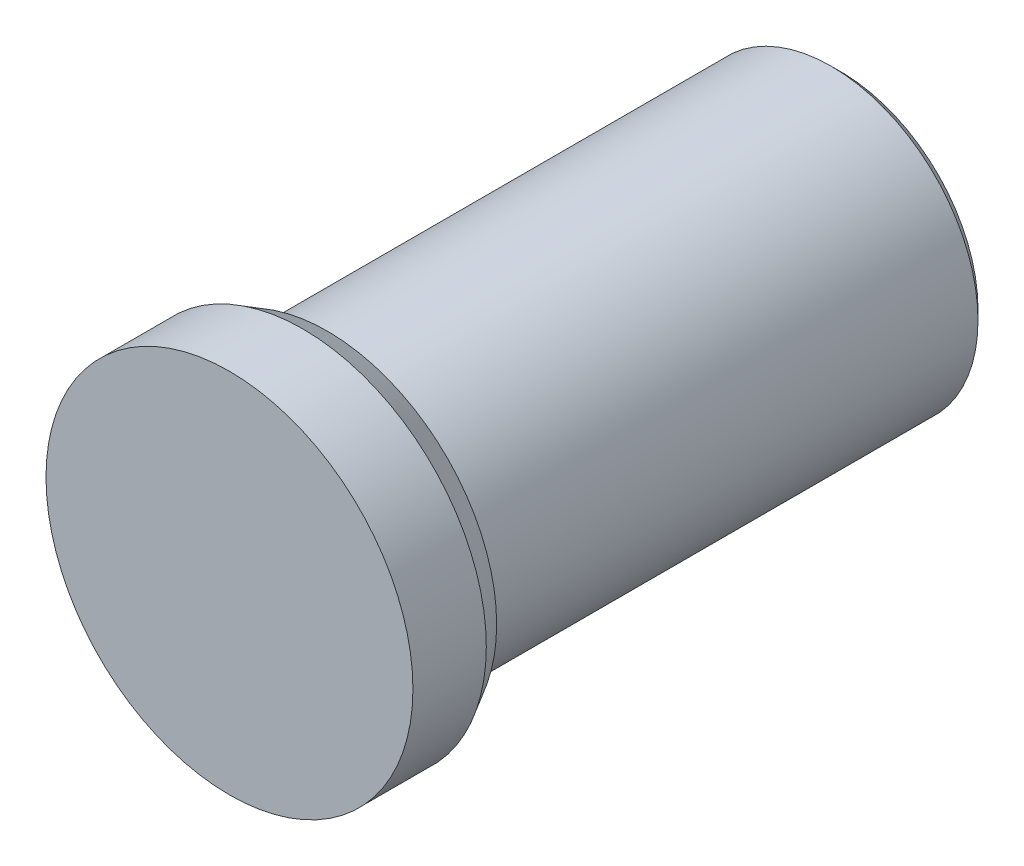
SolidWorks part; units mm, degrees
material "Q345"
ref_plane "前视基准面" through (0, 0, 0) normal (0, 0, 1) x (1, 0, 0)
ref_plane "上视基准面" through (0, 0, 0) normal (0, 1, 0) x (1, 0, 0)
ref_plane "右视基准面" through (0, 0, 0) normal (1, 0, 0) x (0, 0, -1)
sketch "草图1" plane through (0, 0, 0) normal (0, 0, 1) x (1, 0, 0)
  circle A0 centre (0, 0) radius 30
  circle A1 centre (0, 0) radius 20 construction
  dimension "D1" = 60
  dimension "D2" = 40
extrude "凸台-拉伸1" add sketch "草图1" along normal blind 105
sketch "草图2" plane through (0, 0, 105) normal (0, 0, 1) x (1, 0, 0)
  circle A0 centre (0, 0) radius 37.5
  dimension "D1" = 75
extrude "凸台-拉伸2" add sketch "草图2" along normal blind 20
chamfer "倒角2" distance 2 angle 45 1 edges at (30, 0, 0)
ref_axis "基准轴1" through (0, 0, 105) along (0, 0, -1)
sketch "草图3" plane through (0, 0, 0) normal (0, 1, 0) x (1, 0, 0)
  line L1 (30, -105) -> (29, -105)
  line L2 (30, -105) -> (30, -103)
  line L3 (30, -103) -> (29, -103)
  line L4 (29, -105) -> (29, -103)
  dimension "D1" = 2
  dimension "D2" = 1
revolve "切除-旋转1" cut sketch "草图3" angle 360 about axis through (0, 0, 105) along (0, 0, -1)
chamfer "倒角3" distance 5 angle 30 1 edges at (37.5, 0, 105)
